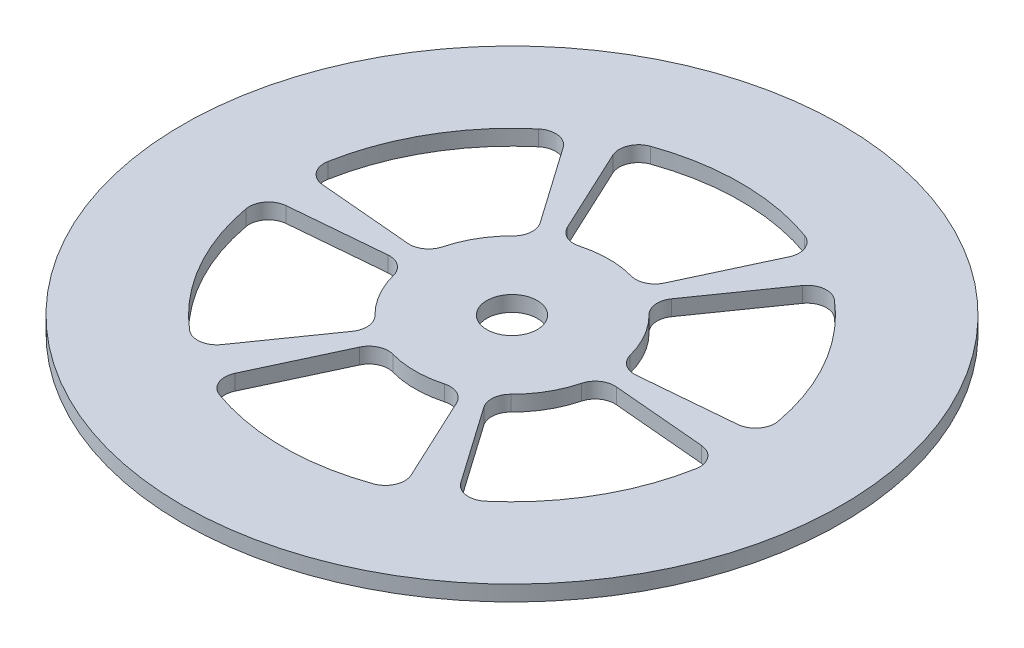
SolidWorks part; units mm, degrees
material "丙烯酸(中高冲击)"
ref_plane "Front Plane" through (0, 0, 0) normal (0, 0, 1) x (1, 0, 0)
ref_plane "Top Plane" through (0, 0, 0) normal (0, 1, 0) x (1, 0, 0)
ref_plane "Right Plane" through (0, 0, 0) normal (1, 0, 0) x (0, 0, -1)
other "Configuration Table"
sketch "Sketch1" plane through (0, 0, 0) normal (0, 1, 0) x (1, 0, 0)
  circle A0 centre (0, 0) radius 85
  circle A1 centre (0, 0) radius 6.5
  point P12 (-3.1161, 0.2799)
  point P16 (0, 0)
  dimension "D1" = 170
  dimension "D2" = 13
extrude "Boss-Extrude1" add sketch "Sketch1" along normal blind 4
sketch "Sketch2" plane through (0, 4, 0) normal (0, 1, 0) x (1, 0, 0)
  line L0 (10.5655, 22.6577) -> (24.9345, 53.4722)
  line L1 (0, 0) -> (0, 53.6207) construction
  line L2 (-10.5655, 22.6577) -> (-24.9345, 53.4722)
  line L3 (14.3394, 20.4788) -> (33.841, 48.33)
  line L4 (24.9049, 2.1789) -> (58.7755, 5.1422)
  line L5 (24.9049, -2.1789) -> (58.7755, -5.1422)
  line L6 (14.3394, -20.4788) -> (33.841, -48.33)
  line L7 (10.5655, -22.6577) -> (24.9345, -53.4722)
  line L8 (-10.5655, -22.6577) -> (-24.9345, -53.4722)
  line L9 (-14.3394, -20.4788) -> (-33.841, -48.33)
  line L10 (-24.9049, -2.1789) -> (-58.7755, -5.1422)
  line L11 (-24.9049, 2.1789) -> (-58.7755, 5.1422)
  line L12 (-14.3394, 20.4788) -> (-33.841, 48.33)
  arc A5 (10.5655, 22.6577) -> (-10.5655, 22.6577) centre (0, 0) ccw
  arc A6 (24.9345, 53.4722) -> (-24.9345, 53.4722) centre (0, 0) ccw
  arc A7 (24.9049, 2.1789) -> (14.3394, 20.4788) centre (0, 0) ccw
  arc A8 (58.7755, 5.1422) -> (33.841, 48.33) centre (0, 0) ccw
  arc A9 (14.3394, -20.4788) -> (24.9049, -2.1789) centre (0, 0) ccw
  arc A10 (33.841, -48.33) -> (58.7755, -5.1422) centre (0, 0) ccw
  arc A11 (-10.5655, -22.6577) -> (10.5655, -22.6577) centre (0, 0) ccw
  arc A12 (-24.9345, -53.4722) -> (24.9345, -53.4722) centre (0, 0) ccw
  arc A13 (-24.9049, -2.1789) -> (-14.3394, -20.4788) centre (0, 0) ccw
  arc A14 (-58.7755, -5.1422) -> (-33.841, -48.33) centre (0, 0) ccw
  arc A15 (-14.3394, 20.4788) -> (-24.9049, 2.1789) centre (0, 0) ccw
  arc A16 (-33.841, 48.33) -> (-58.7755, 5.1422) centre (0, 0) ccw
  point P13 (0, 0)
  point P30 (0, 0)
  dimension "D1" = 50
  dimension "D2" = 118
  dimension "D3" = 25
  dimension "D4" = 6
extrude "Cut-Extrude1" cut sketch "Sketch2" against normal blind 10
fillet "Fillet1" radius 5 24 edges at (10.5655, 2, -22.6577) (-10.5655, 2, -22.6577) (-14.3394, 2, -20.4788) (-24.9049, 2, -2.1789) (-24.9049, 2, 2.1789) (-10.5655, 2, 22.6577) (10.5655, 2, 22.6577) (14.3394, 2, 20.4788) (24.9049, 2, 2.1789) (24.9049, 2, -2.1789) (14.3394, 2, -20.4788) (-14.3394, 2, 20.4788) (-24.9345, 2, 53.4722) (-33.841, 2, 48.33) (-58.7755, 2, 5.1422) (-58.7755, 2, -5.1422) (-33.841, 2, -48.33) (-24.9345, 2, -53.4722) (24.9345, 2, 53.4722) (33.841, 2, 48.33) (58.7755, 2, 5.1422) (58.7755, 2, -5.1422) (33.841, 2, -48.33) (24.9345, 2, -53.4722)
